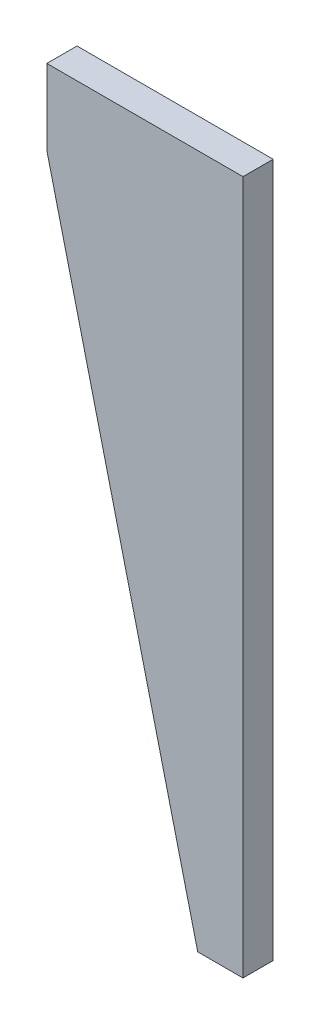
SolidWorks part; units mm, degrees
ref_plane "Front Plane" through (0, 0, 0) normal (0, 0, 1) x (1, 0, 0)
ref_plane "Top Plane" through (0, 0, 0) normal (0, 1, 0) x (1, 0, 0)
ref_plane "Right Plane" through (0, 0, 0) normal (1, 0, 0) x (0, 0, -1)
sketch "Sketch1" plane through (0, 0, 0) normal (0, 0, 1) x (1, 0, 0)
  line L1 (65, -230) -> (-65, -230)
  line L2 (65, -230) -> (65, 230)
  line L3 (65, 230) -> (-65, 230)
  line L4 (-65, -230) -> (-65, 230)
  line L5 (65, -230) -> (-65, 230) construction
  line L6 (65, 230) -> (-65, -230) construction
  point P0 (0, 0)
  dimension "D1" = 130
  dimension "D2" = 460
extrude "Boss-Extrude1" add sketch "Sketch1" along normal mid plane 20
sketch "Sketch2" plane through (0, 0, 10) normal (0, 0, 1) x (1, 0, 0)
  line L0 (-65, 180) -> (35, -230)
  line L1 (-65, 230) -> (-65, -230) construction
  line L2 (-65, -230) -> (65, -230) construction
  line L3 (35, -230) -> (-65, -230)
  line L4 (-65, -230) -> (-65, 180)
  line L5 (65, 230) -> (-65, 230) construction
  line L6 (65, -230) -> (65, 230) construction
  dimension "D1" = 50
  dimension "D2" = 30
extrude "Cut-Extrude1" cut sketch "Sketch2" against normal through all
